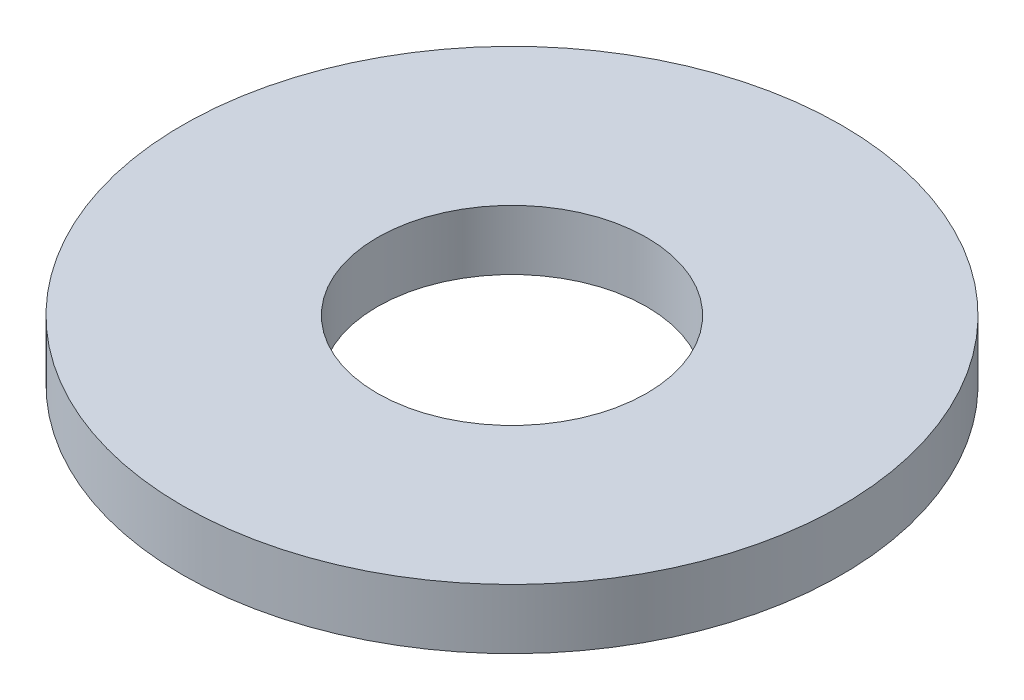
SolidWorks part; units mm, degrees
ref_plane "前视基准面" through (0, 0, 0) normal (0, 0, 1) x (1, 0, 0)
ref_plane "上视基准面" through (0, 0, 0) normal (0, 1, 0) x (1, 0, 0)
ref_plane "右视基准面" through (0, 0, 0) normal (1, 0, 0) x (0, 0, -1)
other "Configuration Table"
sketch "草图1" plane through (0, 0, 0) normal (0, 1, 0) x (1, 0, 0)
  circle A0 centre (0, 0) radius 110
  circle A1 centre (0, 0) radius 45
  dimension "D1" = 220
  dimension "D2" = 90
extrude "凸台-拉伸1" add sketch "草图1" along normal blind 20
